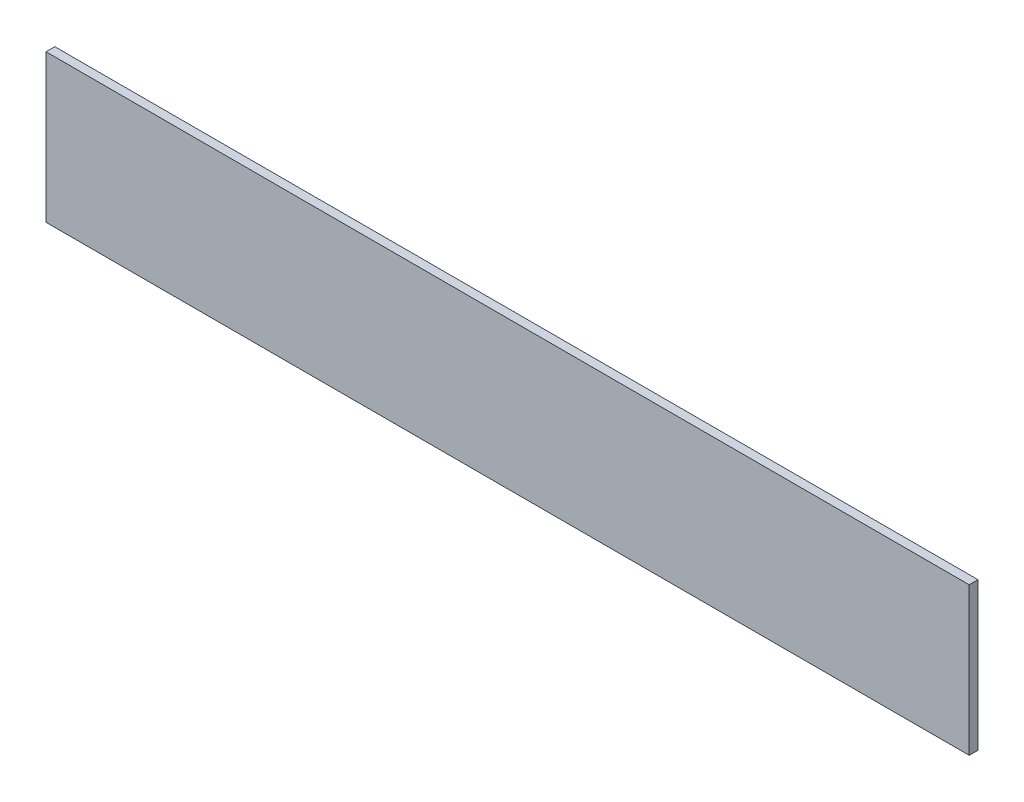
SolidWorks part; units mm, degrees
material "Q235"
ref_plane "Front Plane" through (0, 0, 0) normal (0, 0, 1) x (1, 0, 0)
ref_plane "Top Plane" through (0, 0, 0) normal (0, 1, 0) x (1, 0, 0)
ref_plane "Right Plane" through (0, 0, 0) normal (1, 0, 0) x (0, 0, -1)
sketch "Sketch1" plane through (0, 0, 0) normal (0, 0, 1) x (1, 0, 0)
  line L1 (-1050, 168) -> (1050, 168)
  line L2 (-1050, 168) -> (-1050, -168)
  line L3 (-1050, -168) -> (1050, -168)
  line L4 (1050, 168) -> (1050, -168)
  dimension "D1" = 336
  dimension "D2" = 168
  dimension "D3" = 2100
  dimension "D4" = 1050
extrude "Boss-Extrude1" add sketch "Sketch1" along normal mid plane 20
